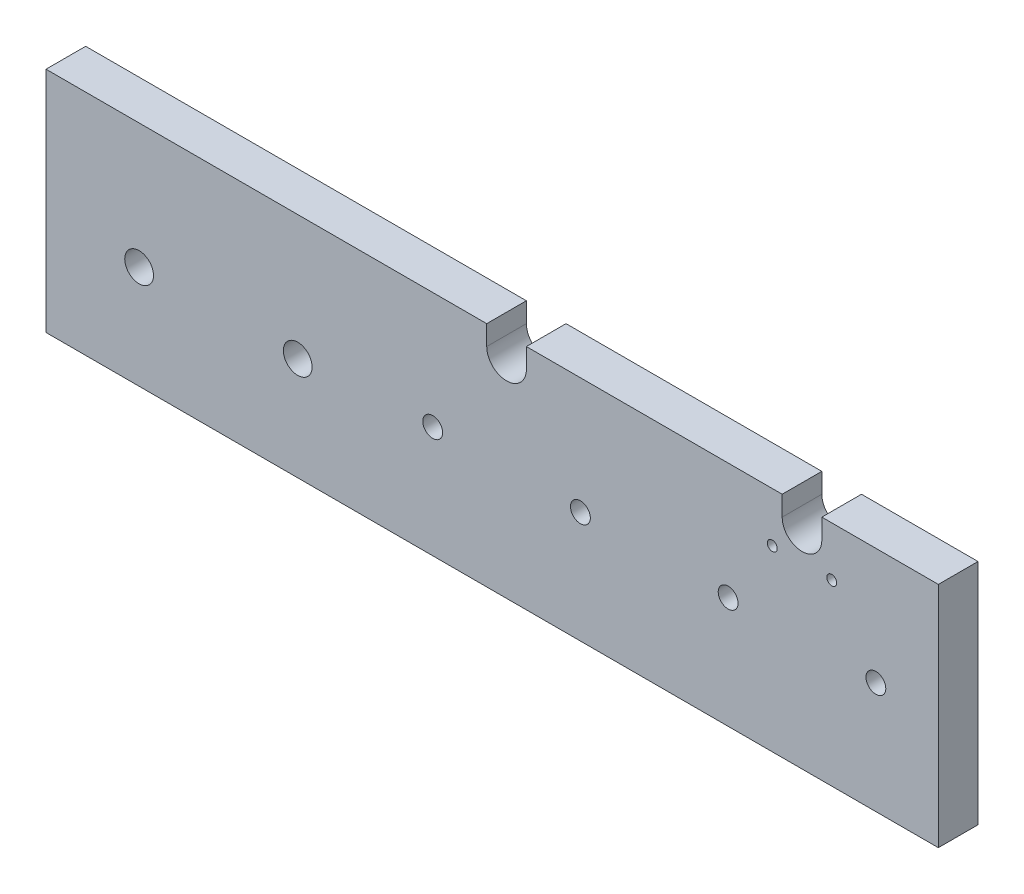
SolidWorks part; units mm, degrees
material "Q235A"
ref_plane "Front Plane" through (0, 0, 0) normal (0, 0, 1) x (1, 0, 0)
ref_plane "Top Plane" through (0, 0, 0) normal (0, 1, 0) x (1, 0, 0)
ref_plane "Right Plane" through (0, 0, 0) normal (1, 0, 0) x (0, 0, -1)
sketch "Sketch1" plane through (0, 0, 0) normal (0, 0, 1) x (1, 0, 0)
  line L1 (450, -115) -> (-450, -115)
  line L2 (450, -115) -> (450, 115)
  line L3 (450, 115) -> (-450, 115)
  line L4 (-450, -115) -> (-450, 115)
  line L5 (450, -115) -> (-450, 115) construction
  line L6 (450, 115) -> (-450, -115) construction
  point P0 (0, 0)
  dimension "D1" = 230
  dimension "D2" = 900
extrude "Boss-Extrude1" add sketch "Sketch1" along normal mid plane 40
sketch "Sketch2" plane through (0, 0, 20) normal (0, 0, 1) x (1, 0, 0)
  line L1 (450, 115) -> (-450, 115) construction
  line L2 (450, -115) -> (450, 115) construction
  circle A0 centre (387, -2.5) radius 10
  dimension "D1" = 20
  dimension "D2" = 63
  dimension "D3" = 117.5
extrude "Cut-Extrude1" cut sketch "Sketch2" against normal through all
sketch "Sketch3" plane through (0, 0, 20) normal (0, 0, 1) x (1, 0, 0)
  line L0 (312.5, 115) -> (312.5, 95) construction
  line L1 (450, 115) -> (-450, 115) construction
  line L2 (332.5, 115) -> (332.5, 95)
  line L3 (292.5, 115) -> (292.5, 95)
  arc A0 (332.5, 115) -> (292.5, 115) centre (312.5, 115) ccw
  arc A1 (292.5, 95) -> (332.5, 95) centre (312.5, 95) ccw
  circle A2 centre (387, -2.5) radius 10 construction
  point P4 (312.5, 105)
  dimension "D1" = 20
  dimension "D3" = 74.5
  dimension "D2" = 20
extrude "Cut-Extrude2" cut sketch "Sketch3" against normal through all
pattern_linear "LPattern1" count 2 spacing 298 along (-1, 0, 0) of "Cut-Extrude2"
pattern_linear "LPattern2" count 4 spacing 149 along (-1, 0, 0) of "Cut-Extrude1"
sketch "Sketch5" plane through (0, 0, -20) normal (0, 0, -1) x (-1, 0, 0)
  line L0 (-312.5, 75) -> (-312.5, -70.3065) construction
  line L1 (-450, 115) -> (-332.5, 115) construction
  circle A0 centre (-342.5, 65) radius 5
  arc A1 (-332.5, 95) -> (-292.5, 95) centre (-312.5, 95) ccw construction
  circle A2 centre (-282.5, 65) radius 5
  dimension "D1" = 10
  dimension "D2" = 50
  dimension "D3" = 60
extrude "Cut-Extrude4" cut sketch "Sketch5" against normal through all
ref_plane "Plane1" through (312.5, 0, 0) normal (-1, 0, 0) x (0, 0, 1)
sketch "Sketch6" plane through (0, 0, -20) normal (0, 0, -1) x (-1, 0, 0)
  line L0 (450, 115) -> (450, -115) construction
  line L1 (5.5, 115) -> (450, 115) construction
  circle A0 centre (356.1, -11) radius 14.5
  circle A1 centre (196.1, -11) radius 14.5
  dimension "D3" = 29
  dimension "D4" = 160
  dimension "D1" = 93.9
  dimension "D2" = 126
extrude "Cut-Extrude5" cut sketch "Sketch6" against normal through all
